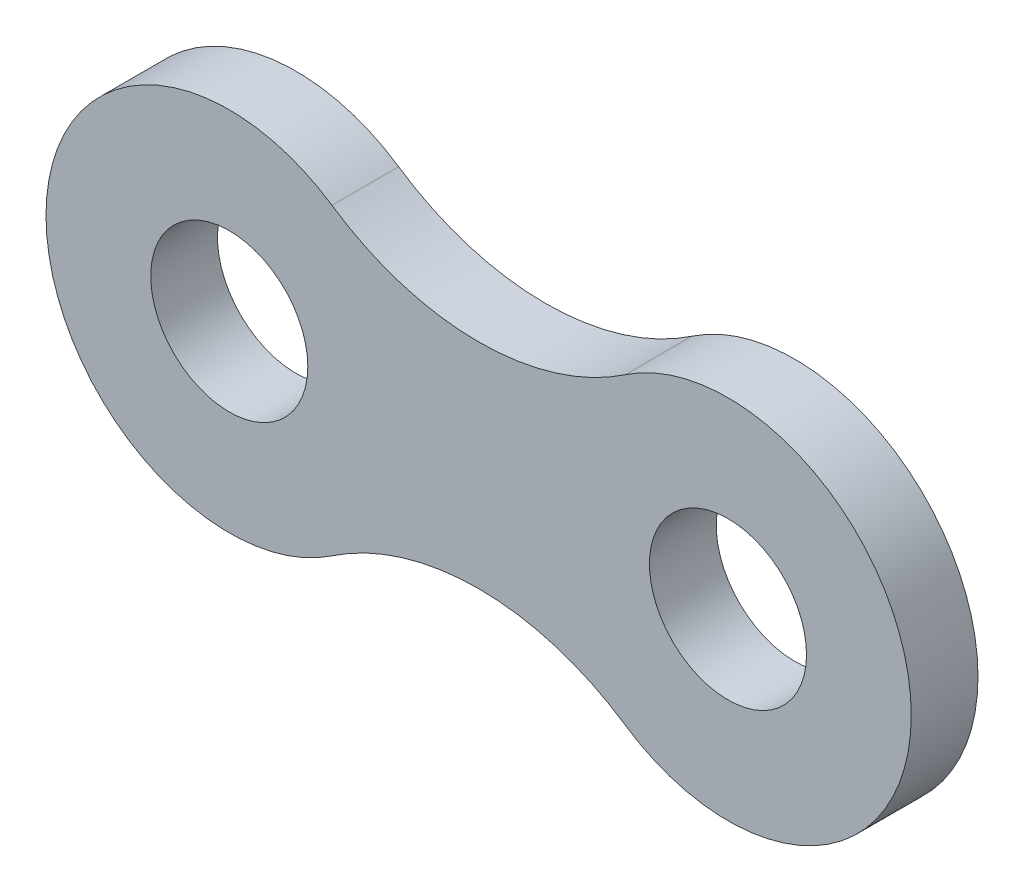
SolidWorks part; units mm, degrees
material "65Mn"
ref_plane "Front Plane" through (0, 0, 0) normal (0, 0, 1) x (1, 0, 0)
ref_plane "Top Plane" through (0, 0, 0) normal (0, 1, 0) x (1, 0, 0)
ref_plane "Right Plane" through (0, 0, 0) normal (1, 0, 0) x (0, 0, -1)
sketch "Sketch1" plane through (0, 0, 0) normal (0, 0, 1) x (1, 0, 0)
  line L0 (0, 0) -> (19.05, 0) construction
  arc A0 (3.9221, 5.7981) -> (3.9221, -5.7981) centre (0, 0) ccw
  arc A1 (15.1279, -5.7981) -> (15.1279, 5.7981) centre (19.05, 0) ccw
  circle A2 centre (0, 0) radius 3
  circle A3 centre (19.05, 0) radius 3
  arc A4 (3.9221, 5.7981) -> (15.1279, 5.7981) centre (9.525, 14.081) ccw
  arc A5 (3.9221, -5.7981) -> (15.1279, -5.7981) centre (9.525, -14.081) cw
  dimension "D1" = 14
  dimension "D2" = 14
  dimension "D4" = 6
  dimension "D5" = 6
  dimension "D6" = 10
  dimension "D3" = 19.05
extrude "Boss-Extrude1" add sketch "Sketch1" along normal blind 2.55
